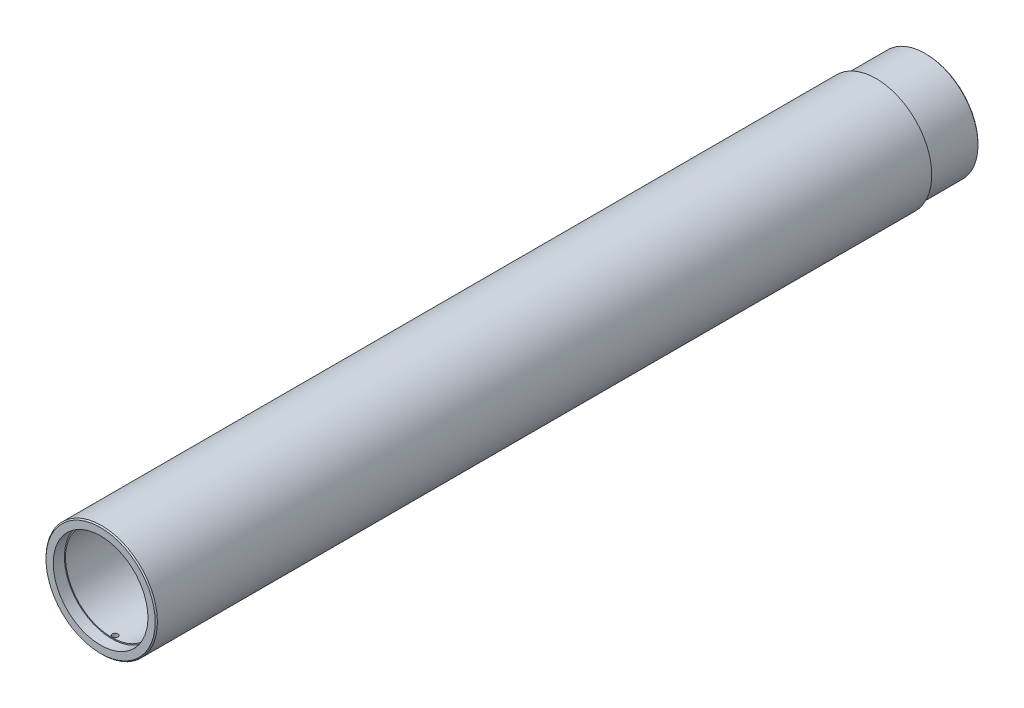
from build123d import *

# Parameters (mm, degrees)
SKETCH1_R             = 50
SKETCH1_R_2           = 40
BOSS_EXTRUDE1_DEPTH   = 741
SKETCH2_R             = 61.681035311
SKETCH2_R_2           = 47.5
CUT_EXTRUDE1_DEPTH    = 45
CHAMFER1_SIZE         = 1
CHAMFER2_SIZE         = 1
SKETCH10_R            = 42.5
CUT_EXTRUDE9_DEPTH    = 10
SKETCH11_R            = 41.5
CUT_EXTRUDE10_DEPTH   = 50
M6_TAPPED_HOLE1_D     = 5
M6_TAPPED_HOLE1_DEPTH = 15
M6_TAPPED_HOLE1_TIP   = 1.502151548


with BuildPart() as part:
    # Sketch1 → Boss-Extrude1 (new body)
    with BuildSketch(Plane.XY):
        Circle(SKETCH1_R)
        Circle(SKETCH1_R_2, mode=Mode.SUBTRACT)
    extrude(amount=BOSS_EXTRUDE1_DEPTH)

    # Sketch2 → Cut-Extrude1 (cut)
    with BuildSketch(Plane(origin=(0, 0, 0), x_dir=(-1, 0, 0), z_dir=(0, 0, -1))):
        Circle(SKETCH2_R)
        Circle(SKETCH2_R_2, mode=Mode.SUBTRACT)
    extrude(amount=-CUT_EXTRUDE1_DEPTH, mode=Mode.SUBTRACT)

    # Chamfer1
    chamfer1_edges = [part.edges().sort_by_distance(p)[0] for p in [
        (47.5, 0, 0),
    ]]
    chamfer(chamfer1_edges, length=CHAMFER1_SIZE)

    # Chamfer2
    chamfer2_edges = [part.edges().sort_by_distance(p)[0] for p in [
        (-50, 0, 741),
    ]]
    chamfer(chamfer2_edges, length=CHAMFER2_SIZE)

    # Sketch10 → Cut-Extrude9 (cut)
    with BuildSketch(Plane.XY.offset(741)):
        Circle(SKETCH10_R)
    extrude(amount=-CUT_EXTRUDE9_DEPTH, mode=Mode.SUBTRACT)

    # Sketch11 → Cut-Extrude10 (cut)
    with BuildSketch(Plane.XY.offset(731)):
        Circle(SKETCH11_R)
    extrude(amount=-CUT_EXTRUDE10_DEPTH, mode=Mode.SUBTRACT)

    # M6 Tapped Hole1
    with Locations(Plane.XZ.offset(50)):
        with Locations((0, 728)):
            Hole(M6_TAPPED_HOLE1_D / 2, depth=M6_TAPPED_HOLE1_DEPTH)
            with Locations((0, 0, -(M6_TAPPED_HOLE1_DEPTH + M6_TAPPED_HOLE1_TIP / 2))):  # 118° drill point
                Cone(0, M6_TAPPED_HOLE1_D / 2, M6_TAPPED_HOLE1_TIP, mode=Mode.SUBTRACT)


solid = part.part
